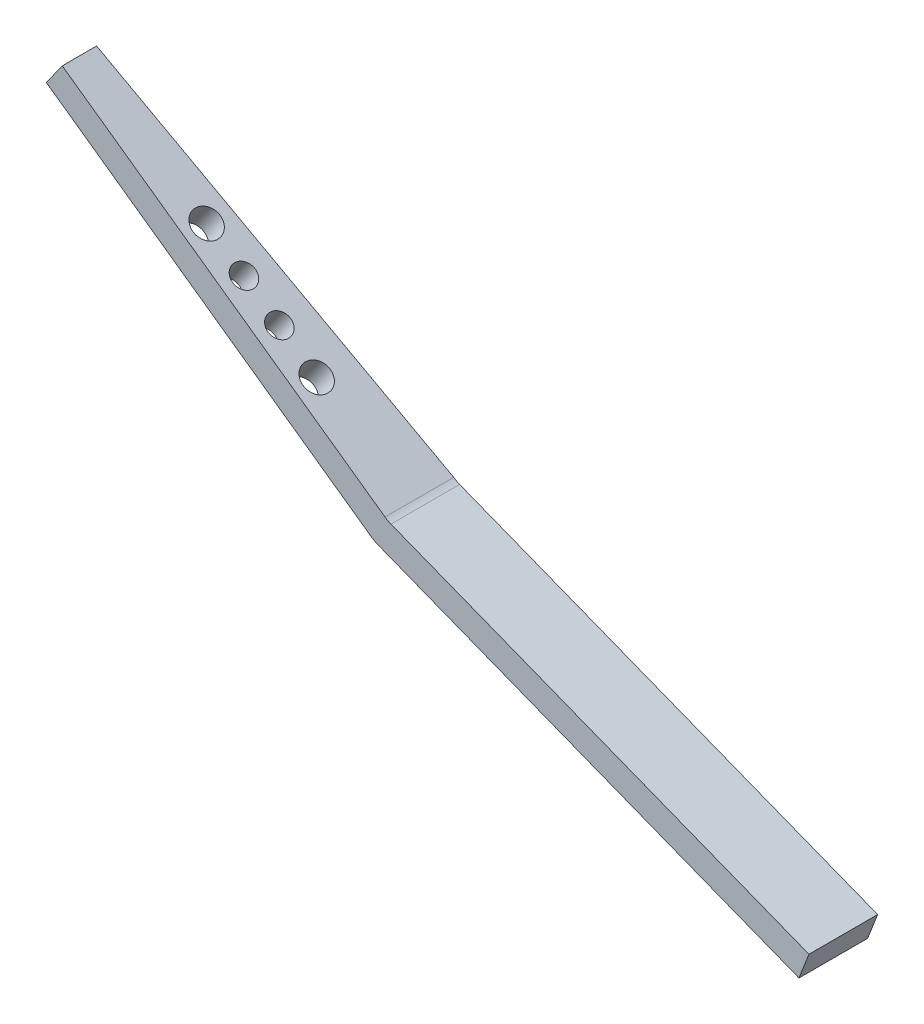
SolidWorks part; units mm, degrees
ref_plane "前视基准面" through (0, 0, 0) normal (0, 0, 1) x (1, 0, 0)
ref_plane "上视基准面" through (0, 0, 0) normal (0, 1, 0) x (1, 0, 0)
ref_plane "右视基准面" through (0, 0, 0) normal (1, 0, 0) x (0, 0, -1)
sketch "草图1" plane through (0, 0, 0) normal (0, 0, 1) x (1, 0, 0)
  line L0 (-156.5525, 182.2852) -> (-144.9682, 198.5887) construction
  line L1 (13.8693, 98.0078) -> (19.1595, 111.5352) construction
  line L2 (-70.4205, 151.9363) -> (16.324, 118.0128) construction
  line L3 (-137.9962, 199.7685) -> (-71.4955, 152.517) construction
  line L4 (-145.5474, 197.7735) -> (-142.0721, 202.6646)
  line L5 (18.7953, 110.6039) -> (20.9806, 116.1918)
  line L6 (-70.3058, 151.8914) -> (20.9806, 116.1918)
  line L7 (-142.0721, 202.6646) -> (-71.5958, 152.5883)
  line L8 (-145.5474, 197.7735) -> (-74.469, 147.2694)
  line L9 (-73.179, 146.5726) -> (18.7953, 110.6039)
  line L12 (-141.4715, 194.8775) -> (-74.9708, 147.6259) construction
  line L13 (-137.9962, 199.7685) -> (-71.4955, 152.517) construction
  line L14 (-70.4205, 151.9363) -> (16.324, 118.0128) construction
  line L15 (-72.6058, 146.3484) -> (14.1387, 112.425) construction
  arc A0 (-73.179, 146.5726) -> (-74.469, 147.2694) centre (-70.9937, 152.1605) cw
  arc A1 (-70.3058, 151.8914) -> (-71.5958, 152.5883) centre (-68.1206, 157.4793) cw
  dimension "D1" = 6
  dimension "D2" = 6
ref_plane "基准面4" through (-137.9962, 199.7685, 0) normal (0.8152, -0.5792, 0) x (0, 0, -1)
extrude "凸台-拉伸1" add sketch "草图1" along normal blind 15
sketch "草图3" plane through (48.0266, 67.5916, 0) normal (0.5792, 0.8152, 0) x (0.8152, -0.5792, 0)
  line L0 (-233.2, -7.5) -> (-172.4387, -15)
  line L1 (-233.2, -15) -> (-233.2, 0) construction
  line L2 (-146.7446, -15) -> (-233.2, -15) construction
  line L3 (-172.4387, -15) -> (-172.9644, -27.6527)
  line L4 (-172.9644, -27.6527) -> (-246.3137, -29.0154)
  line L5 (-246.3137, -29.0154) -> (-233.2, -7.5)
sketch "草图4" plane through (48.0266, 67.5916, 0) normal (0.5792, 0.8152, 0) x (0.8152, -0.5792, 0)
  line L0 (-233.2, -7.5) -> (-146.7446, 0)
  line L1 (-233.2, -15) -> (-233.2, 0) construction
  line L2 (-146.7446, 0) -> (-233.2, 0)
  line L3 (-233.2, 0) -> (-233.2, -7.5)
extrude "切除-拉伸1" cut sketch "草图4" against normal through all
sketch "草图5" plane through (48.0266, 67.5916, 0) normal (0.5792, 0.8152, 0) x (0.8152, -0.5792, 0)
  ellipse E0 centre (-171.0199, -10.1292) end of major axis (-171.0199, -13.1292) minor radius 2.9999 construction
  ellipse E1 centre (-200.5026, -10.1292) end of major axis (-200.5026, -13.1292) minor radius 2.9999 construction
  ellipse E2 centre (-171.0199, -10.1292) end of major axis (-171.0199, -13.1292) minor radius 2.9999
  ellipse E3 centre (-200.5026, -10.1292) end of major axis (-200.5026, -13.1292) minor radius 2.9999
extrude "切除-拉伸2" cut sketch "草图5" against normal through all
hole_wizard "M6 螺纹孔1" positions "草图6" profile "草图7" tap size "M6" standard "GB" end condition through all
sketch "草图6" plane through (48.0266, 67.5916, 0) normal (0.5792, 0.8152, 0) x (0.8152, -0.5792, 0)
  point P0 (-181.0197, -10.1292)
  point P4 (-190.5028, -10.1292)
sketch "草图7" plane through (-99.536, 172.4409, 10.1292) normal (0, 0, 1) x (-0.8152, 0.5792, 0)
  line L0 (0, 0) -> (0, 77.0585)
  line L1 (0, 77.0585) -> (2.5, 77.0585)
  line L2 (2.5, 77.0585) -> (2.5, 0)
  line L5 (2.5, 0) -> (0, 0)
  line L11 (0, -6.35) -> (0, 107.95) construction
  dimension "通孔螺纹孔钻头直径" = 5
  dimension "通孔螺纹孔钻头深度" = 77.0585
cosmetic thread "孔螺蚊线1" parameters "D2"=6
cosmetic thread "孔螺蚊线2" parameters "D2"=6
